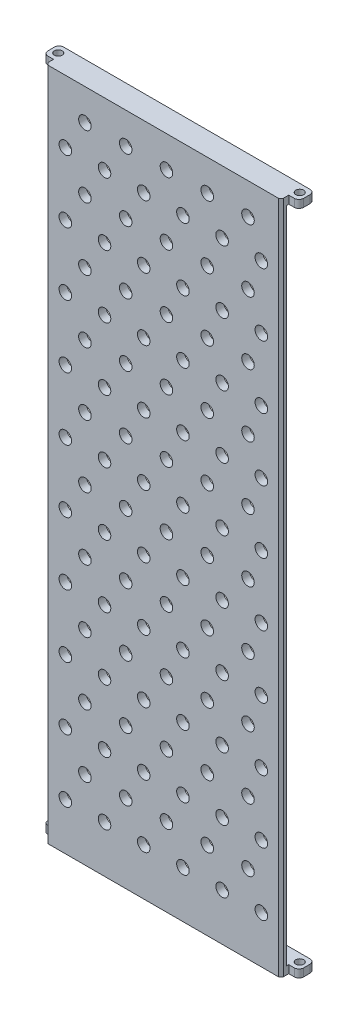
SolidWorks part; units mm, degrees
ref_plane "Front Plane" through (0, 0, 0) normal (0, 0, 1) x (1, 0, 0)
ref_plane "Top Plane" through (0, 0, 0) normal (0, 1, 0) x (1, 0, 0)
ref_plane "Right Plane" through (0, 0, 0) normal (1, 0, 0) x (0, 0, -1)
other "Configuration Table"
sketch "Sketch1" plane through (0, 0, 0) normal (0, 0, 1) x (1, 0, 0)
  line L1 (0, 0) -> (150, 0)
  line L2 (0, 0) -> (0, 420)
  line L3 (0, 420) -> (150, 420)
  line L4 (150, 0) -> (150, 420)
  dimension "D1" = 420
  dimension "D2" = 150
extrude "Boss-Extrude1" add sketch "Sketch1" along normal blind 5
sketch "Sketch2" plane through (0, 0, 5) normal (0, 0, 1) x (1, 0, 0)
  line L0 (0, 405) -> (150, 405) construction
  line L1 (0, 420) -> (0, 0) construction
  line L2 (150, 0) -> (150, 420) construction
  line L3 (0, 385) -> (150, 385) construction
  line L4 (150, 420) -> (0, 420) construction
  line L5 (25, 420) -> (25, 385) construction
  line L6 (12.5, 420) -> (12.5, 385) construction
  line L7 (12.5, 385) -> (37.5, 385) construction
  circle A0 centre (25, 405) radius 4
  circle A1 centre (51, 405) radius 4
  circle A2 centre (77, 405) radius 4
  circle A3 centre (103, 405) radius 4
  circle A4 centre (129, 405) radius 4
  circle A5 centre (12.5, 385) radius 4
  circle A6 centre (37.5, 385) radius 4
  circle A7 centre (62.5, 385) radius 4
  circle A8 centre (87.5, 385) radius 4
  circle A9 centre (112.5, 385) radius 4
  circle A10 centre (137.5, 385) radius 4
  dimension "D3" = 8
  dimension "D7" = 8
  dimension "D1" = 15
  dimension "D2" = 20
  dimension "D4" = 25
  dimension "D6" = 12.5
  dimension "D9" = 25
  dimension "D5" = 5
  dimension "D8" = 6
extrude "Cut-Extrude1" cut sketch "Sketch2" against normal up to next
pattern_linear "LPattern1" count 10 spacing 40 along (0, -1, 0) of "Cut-Extrude1"
sketch "Sketch3" plane through (0, 0, 0) normal (0, -1, 0) x (-1, 0, 0)
  line L0 (0, -5) -> (-150, -5) construction
  line L1 (6.5, 10) -> (-156.5, 10)
  line L2 (6.5, 10) -> (6.5, 0)
  line L3 (0, -5) -> (-150, -5)
  line L4 (-156.5, 10) -> (-156.5, 0)
  line L5 (0, -5) -> (0, 0) construction
  line L6 (-150, 0) -> (-150, -5)
  line L7 (-150, 0) -> (-156.5, 0)
  line L8 (0, -5) -> (0, 0)
  line L9 (0, 0) -> (6.5, 0)
  dimension "D2" = 163
  dimension "D3" = 0
  dimension "D4" = 6.5
  dimension "D5" = 5
extrude "Boss-Extrude2" add sketch "Sketch3" along normal blind 5
sketch "Sketch4" plane through (0, 420, 0) normal (0, 1, 0) x (1, 0, 0)
  line L0 (150, -5) -> (150, 0)
  line L5 (-6.5, 10) -> (156.5, 10)
  line L6 (-6.5, 10) -> (-6.5, 0)
  line L7 (0, -5) -> (150, -5)
  line L8 (156.5, 10) -> (156.5, 0)
  line L9 (150, 0) -> (156.5, 0)
  line L10 (0, -5) -> (0, 0)
  line L11 (0, 0) -> (-6.5, 0)
extrude "Boss-Extrude3" add sketch "Sketch4" along normal blind 5
sketch "Sketch6" plane through (0, 425, 0) normal (0, 1, 0) x (1, 0, 0)
  line L0 (156.5, 0) -> (156.5, 10) construction
  line L1 (-6.5, 10) -> (-6.5, 0) construction
  line L2 (156.5, 10) -> (-6.5, 10) construction
  line L4 (150, -5) -> (156.5, -5)
  line L5 (150, -5) -> (150, 0)
  line L6 (150, 0) -> (156.5, 0)
  line L7 (156.5, -5) -> (156.5, 0)
  line L8 (0, -5) -> (-6.5, -5)
  line L9 (0, -5) -> (0, 0)
  line L10 (0, 0) -> (-6.5, 0)
  line L11 (-6.5, -5) -> (-6.5, 0)
  circle A0 centre (-2, 5) radius 2.5
  circle A1 centre (152, 5) radius 2.5
  dimension "D1" = 4.5
  dimension "D2" = 5
  dimension "D3" = 5
  dimension "D4" = 4.5
  dimension "D5" = 5
  dimension "D6" = 5
extrude "Cut-Extrude2" cut sketch "Sketch6" against normal through all both and the other way through all
fillet "Fillet1" radius 3 8 edges at (-6.5, -2.5, -10) (-6.5, 422.5, -10) (156.5, 422.5, -10) (156.5, -2.5, -10) (-6.5, -2.5, 0) (156.5, -2.5, 0) (156.5, 422.5, 0) (-6.5, 422.5, 0)
chamfer "Chamfer1" distance 1.5 angle 45 4 edges at (0, 210, 5) (0, 210, 0) (150, 210, 5) (150, 210, 0)
